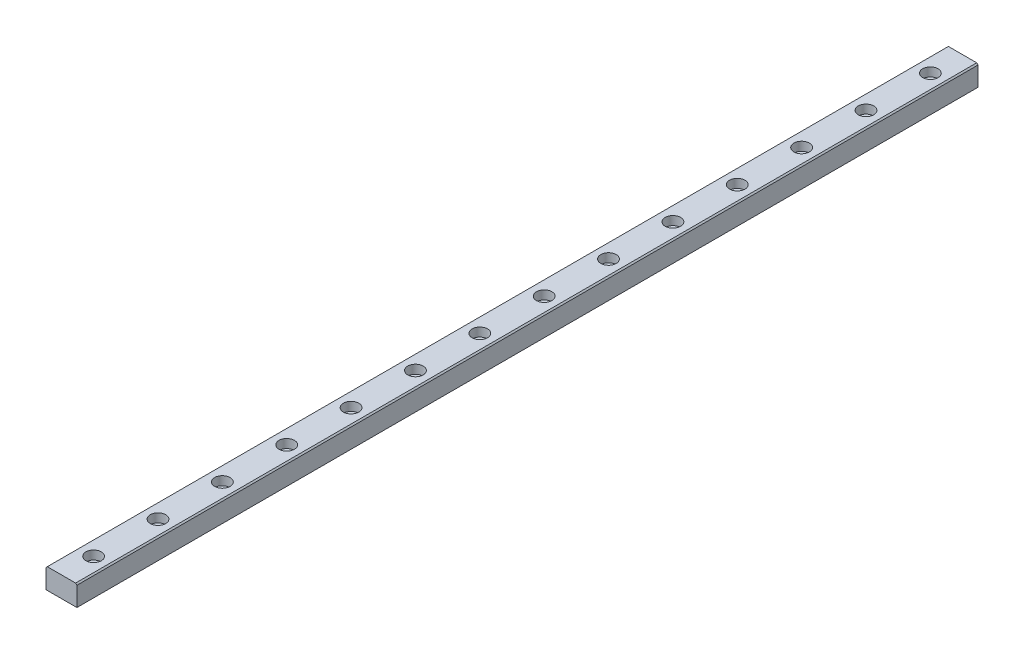
from build123d import *

# Parameters (mm, degrees)
SKETCH_1_W                = 12
SKETCH_1_H                = 8
EXTRUDE_1_DEPTH           = 350
CHAMFER_1_SIZE            = 0.5
CHAMFER_2_SIZE            = 0.5
HOLE_WIZARD_1_D           = 3.4
HOLE_WIZARD_1_CBORE_D     = 6
HOLE_WIZARD_1_CBORE_DEPTH = 3.4
PATTERN_LINEAR_1_COUNT    = 14
PATTERN_LINEAR_1_PITCH    = 25


with BuildPart() as part:
    # 草图1 → 凸台-拉伸1 (new body)
    with BuildSketch(Plane.XY):
        Rectangle(SKETCH_1_W, SKETCH_1_H)
    extrude(amount=EXTRUDE_1_DEPTH)

    # 倒角1
    chamfer_1_edges = [part.edges().sort_by_distance(p)[0] for p in [
        (6, 4, 175),
    ]]
    chamfer(chamfer_1_edges, length=CHAMFER_1_SIZE)

    # 倒角2
    chamfer_2_edges = [part.edges().sort_by_distance(p)[0] for p in [
        (-6, 4, 175),
    ]]
    chamfer(chamfer_2_edges, length=CHAMFER_2_SIZE)

    # 打孔尺寸根据内六角圆柱头螺钉的类型1 (through all)
    with Locations(Plane(origin=(0, 4, 0), x_dir=(1, 0, 0), z_dir=(0, 1, 0))):
        with Locations((0, -12.5)):
            hole_wizard_1 = CounterBoreHole(HOLE_WIZARD_1_D / 2, HOLE_WIZARD_1_CBORE_D / 2, HOLE_WIZARD_1_CBORE_DEPTH)

    # 阵列(线性)1: 打孔尺寸根据内六角圆柱头螺钉的类型1 ×14
    with Locations(*[(0, 0, i * PATTERN_LINEAR_1_PITCH) for i in range(1, PATTERN_LINEAR_1_COUNT)]):
        add(hole_wizard_1, mode=Mode.SUBTRACT)


solid = part.part
